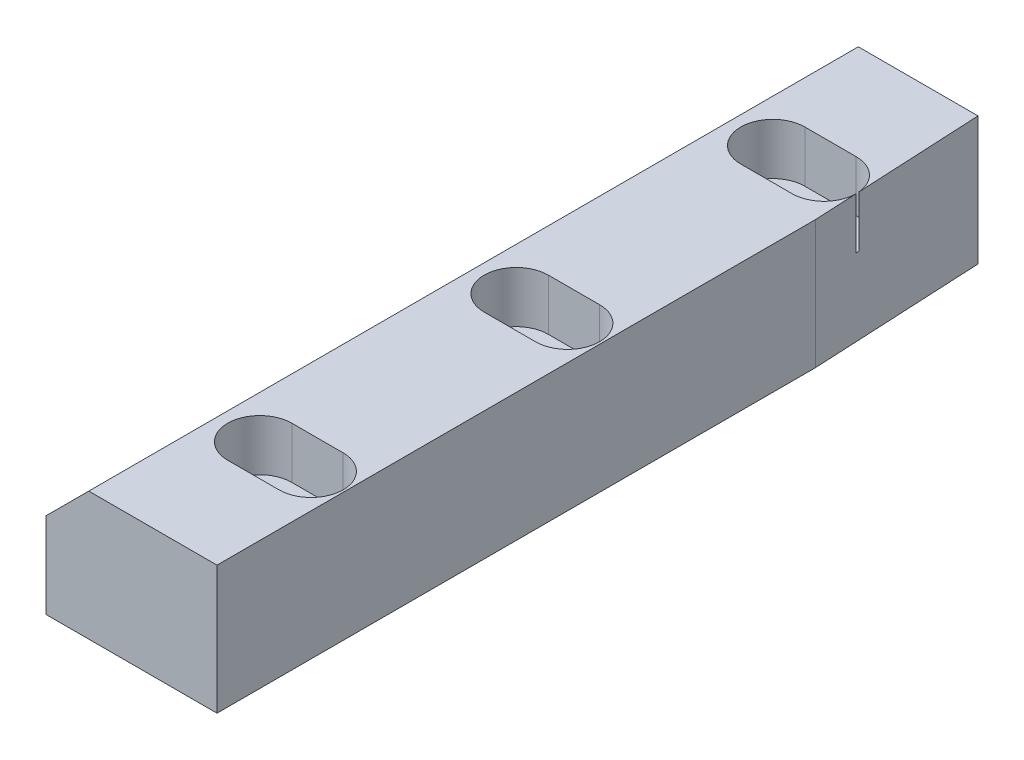
from build123d import *

# Parameters (mm, degrees)
SKETCH1_W                 = 20
SKETCH1_H                 = 90
BOSS_EXTRUDE1_DEPTH       = 15
CHAMFER1_SIZE             = 5
CUT_EXTRUDE1_DEPTH        = 49.476798574
CUT_EXTRUDE2_DEPTH        = 49.476798574
CUT_EXTRUDE3_DEPTH        = 6
LINEAR_PATTERN1_COUNT     = 2
LINEAR_PATTERN1_PITCH     = 30
LINEAR_PATTERN1_COL_COUNT = 2
LINEAR_PATTERN1_COL_PITCH = 30


with BuildPart() as part:
    # Sketch1 → Boss-Extrude1 (new body)
    with BuildSketch(Plane(origin=(0, 0, 0), x_dir=(1, 0, 0), z_dir=(0, 1, 0))):
        Rectangle(SKETCH1_W, SKETCH1_H)
    extrude(amount=BOSS_EXTRUDE1_DEPTH)

    # Chamfer1
    chamfer1_edges = [part.edges().sort_by_distance(p)[0] for p in [
        (-10, 15, 0),
    ]]
    chamfer(chamfer1_edges, length=CHAMFER1_SIZE)

    # Sketch2 → Cut-Extrude1 (cut, through all)
    with BuildSketch(Plane(origin=(0, 15, 0), x_dir=(1, 0, 0), z_dir=(0, 1, 0))):
        Polygon((10, 25), (9, 45), (10, 45), align=None)
    extrude(amount=-CUT_EXTRUDE1_DEPTH, mode=Mode.SUBTRACT)

    # Sketch3 → Cut-Extrude2 (cut, through all)
    with BuildSketch(Plane(origin=(0, 15, 0), x_dir=(1, 0, 0), z_dir=(0, 1, 0))):
        with BuildLine():
            Line((0, 2.25), (6, 2.25))
            ThreePointArc((6, 2.25), (8.25, 0), (6, -2.25))
            Line((6, -2.25), (0, -2.25))
            ThreePointArc((0, -2.25), (-2.25, 0), (0, 2.25))
        make_face()
    cut_extrude2 = extrude(amount=-CUT_EXTRUDE2_DEPTH, mode=Mode.SUBTRACT)

    # Sketch4 → Cut-Extrude3 (cut)
    with BuildSketch(Plane(origin=(0, 15, 0), x_dir=(1, 0, 0), z_dir=(0, 1, 0))):
        with BuildLine():
            Line((0, -3.75), (6, -3.75))
            ThreePointArc((6, -3.75), (9.75, 0), (6, 3.75))
            Line((6, 3.75), (0, 3.75))
            ThreePointArc((0, 3.75), (-3.75, 0), (0, -3.75))
        make_face()
    cut_extrude3 = extrude(amount=-CUT_EXTRUDE3_DEPTH, mode=Mode.SUBTRACT)

    # Linear pattern1: Cut-Extrude2, Cut-Extrude3 ×2
    with Locations(*[(0, 0, i * LINEAR_PATTERN1_PITCH) for i in range(1, LINEAR_PATTERN1_COUNT)]):
        add(cut_extrude2, mode=Mode.SUBTRACT)
        add(cut_extrude3, mode=Mode.SUBTRACT)

    # Linear pattern1 col: Cut-Extrude2, Cut-Extrude3 ×2
    with Locations(*[(0, 0, -i * LINEAR_PATTERN1_COL_PITCH) for i in range(1, LINEAR_PATTERN1_COL_COUNT)]):
        add(cut_extrude2, mode=Mode.SUBTRACT)
        add(cut_extrude3, mode=Mode.SUBTRACT)


solid = part.part
